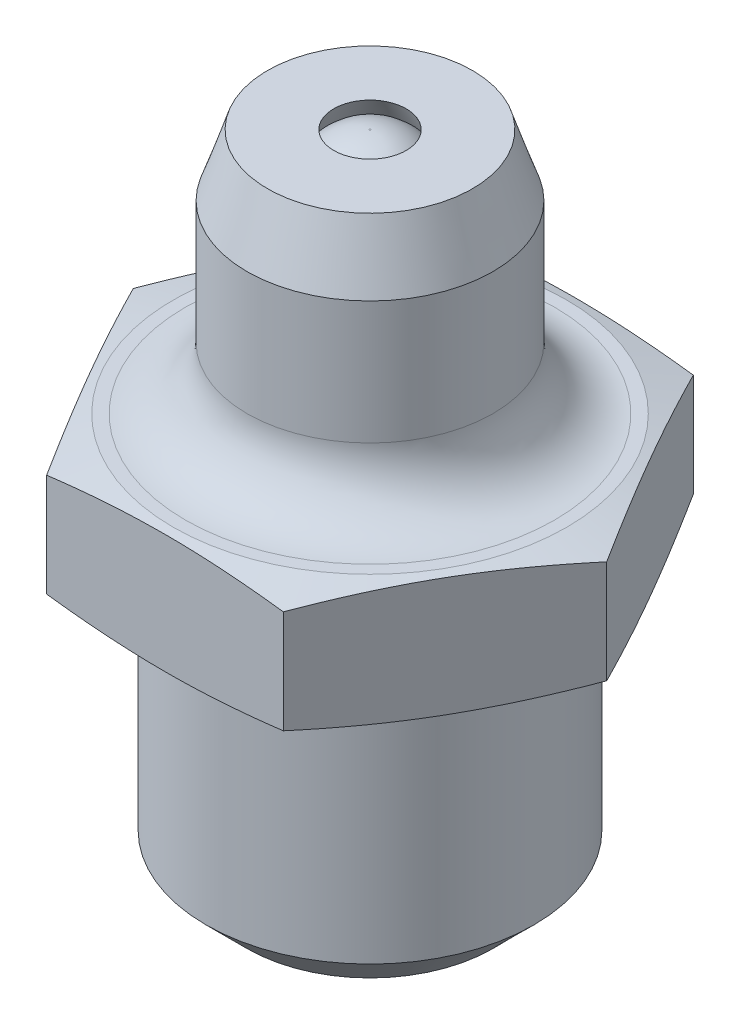
from build123d import *

# Parameters (mm, degrees)
SKETCH1_R           = 4
BOSS_EXTRUDE1_DEPTH = 6.8
BOSS_EXTRUDE2_DEPTH = 3
CHAMFER1_SIZE       = 1


with BuildPart() as part:
    # Sketch1 → Boss-Extrude1 (new body)
    with BuildSketch(Plane(origin=(0, 0, 0), x_dir=(1, 0, 0), z_dir=(0, 1, 0))):
        with Locations(Location((0, 0, 0), (0, 0, 270))):
            Circle(SKETCH1_R)
    extrude(amount=BOSS_EXTRUDE1_DEPTH)

    # Sketch2 → Boss-Extrude2 (add)
    with BuildSketch(Plane(origin=(0, 6.8, 0), x_dir=(1, 0, 0), z_dir=(0, 1, 0))):
        Polygon((2.886751346, -5), (5.773502692, 0), (2.886751346, 5), (-2.886751346, 5), (-5.773502692, 0), (-2.886751346, -5), align=None)
    extrude(amount=BOSS_EXTRUDE2_DEPTH)

    # Sketch3 → Revolve1 (revolve)
    with BuildSketch(Plane.XY, mode=Mode.PRIVATE) as revolve1_sk:
        with BuildLine():
            Line((0, 15.8), (0, 9.8))
            Line((0, 9.8), (4.500264384, 9.8))
            ThreePointArc((4.500264384, 9.8), (3.439434496, 10.239233666), (3, 11.29998038))
            Line((3, 11.29998038), (3, 14.3))
            Line((3, 14.3), (2.5, 15.8))
            Line((2.5, 15.8), (0, 15.8))
        make_face()
    revolve(revolve1_sk.sketch.rotate(Axis((0, -1.880404244, 0), (0, 1, 0)), 90), axis=Axis((0, -1.880404244, 0), (0, 1, 0)))

    # Sketch5 → Cut-Revolve1 (revolve, cut)
    with BuildSketch(Plane(origin=(0, 0, 0), x_dir=(0, 0, -1), z_dir=(1, 0, 0)), mode=Mode.PRIVATE) as cut_revolve1_sk:
        Polygon((-6.8, 9.8), (-4.8, 9.8), (-6.8, 9.3), align=None)
        Polygon((-6.8, 7.3), (-4.8, 6.8), (-6.8, 6.8), align=None)
    revolve(cut_revolve1_sk.sketch.rotate(Axis((0, 16.999618754, 0), (0, -1, 0)), 209.999999988), axis=Axis((0, 16.999618754, 0), (0, -1, 0)), mode=Mode.SUBTRACT)

    # Chamfer1
    chamfer1_edges = [part.edges().sort_by_distance(p)[0] for p in [
        (0, 0, -4),
    ]]
    chamfer(chamfer1_edges, length=CHAMFER1_SIZE)

    # Sketch6 → Cut-Revolve4 (revolve, cut)
    with BuildSketch(Plane(origin=(0, 0, 0), x_dir=(0, 0, -1), z_dir=(1, 0, 0))):
        with BuildLine():
            ThreePointArc((-1.292971656, 15.018429463), (-0.764043535, 15.584287943), (-0.02011539, 15.8))
            Line((-0.02011539, 15.8), (-0.882862678, 15.8))
            Line((-0.882862678, 15.8), (-1.292971656, 15.018429463))
        make_face()
    revolve(axis=Axis((0, 16.917153181, 0), (0, -1, 0)), mode=Mode.SUBTRACT)


solid = part.part
